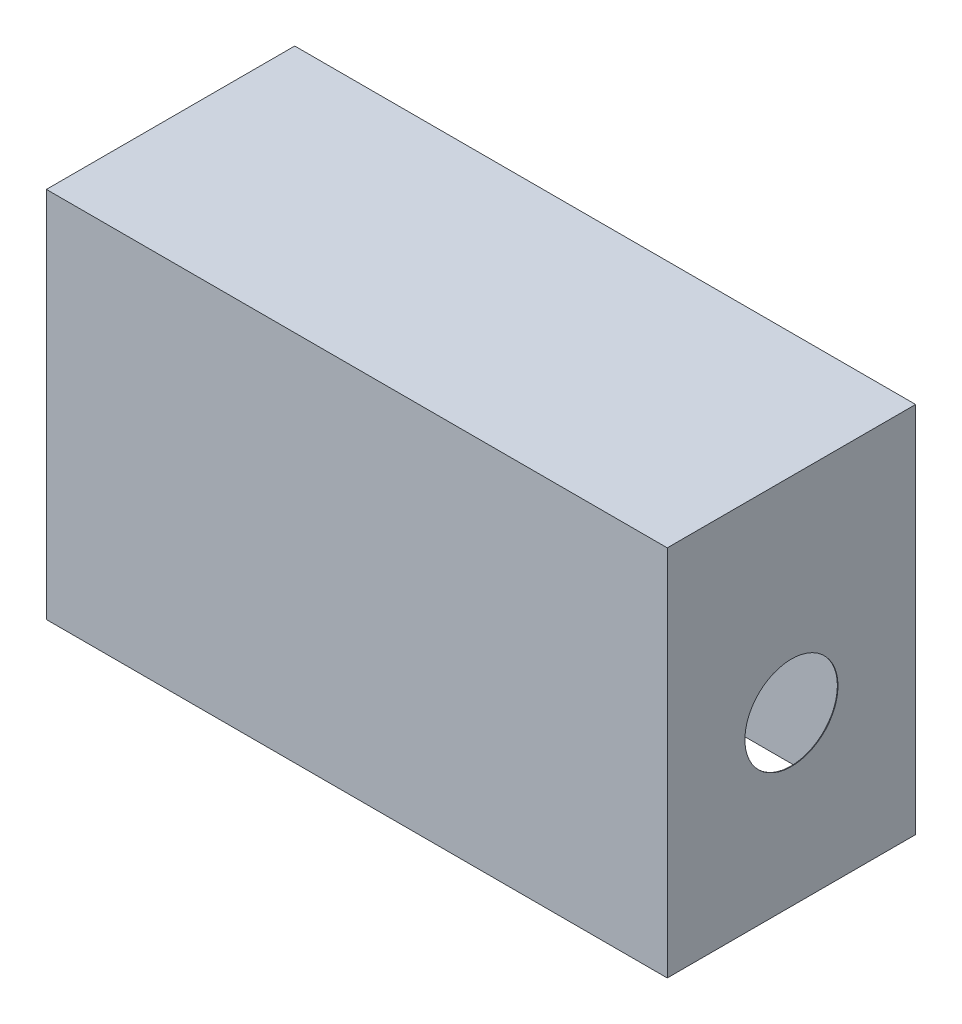
SolidWorks part; units mm, degrees
ref_plane "Front Plane" through (0, 0, 0) normal (0, 0, 1) x (1, 0, 0)
ref_plane "Top Plane" through (0, 0, 0) normal (0, 1, 0) x (1, 0, 0)
ref_plane "Right Plane" through (0, 0, 0) normal (1, 0, 0) x (0, 0, -1)
sketch "Sketch1" plane through (0, 0, 0) normal (0, 1, 0) x (1, 0, 0)
  line L1 (-500, 200) -> (500, 200)
  line L2 (-500, 200) -> (-500, -200)
  line L3 (-500, -200) -> (500, -200)
  line L4 (500, 200) -> (500, -200)
  line L5 (-500, 200) -> (500, -200) construction
  line L6 (-500, -200) -> (500, 200) construction
  point P0 (0, 0)
  dimension "D1" = 1000
  dimension "D2" = 400
extrude "Boss-Extrude1" add sketch "Sketch1" along normal blind 600
sketch "Sketch2" plane through (0, 0, 0) normal (0, -1, 0) x (1, 0, 0)
  line L0 (-500, 200) -> (500, 200) construction
  line L1 (-499, -199) -> (499, -199)
  line L2 (-499, -199) -> (-499, 199)
  line L3 (-499, 199) -> (499, 199)
  line L4 (499, -199) -> (499, 199)
  line L5 (-499, -199) -> (499, 199) construction
  line L6 (-499, 199) -> (499, -199) construction
  line L7 (-500, -200) -> (-500, 200) construction
  point P0 (0, 0)
  dimension "D1" = 1
  dimension "D2" = 1
extrude "Cut-Extrude1" cut sketch "Sketch2" against normal blind 599
sketch "Sketch3" plane through (500, 0, 0) normal (1, 0, 0) x (0, 0, -1)
  line L0 (-200, 0) -> (200, 0) construction
  circle A0 centre (0, 270) radius 75
  dimension "D1" = 150
  dimension "D2" = 270
extrude "Cut-Extrude2" cut sketch "Sketch3" against normal blind 50
